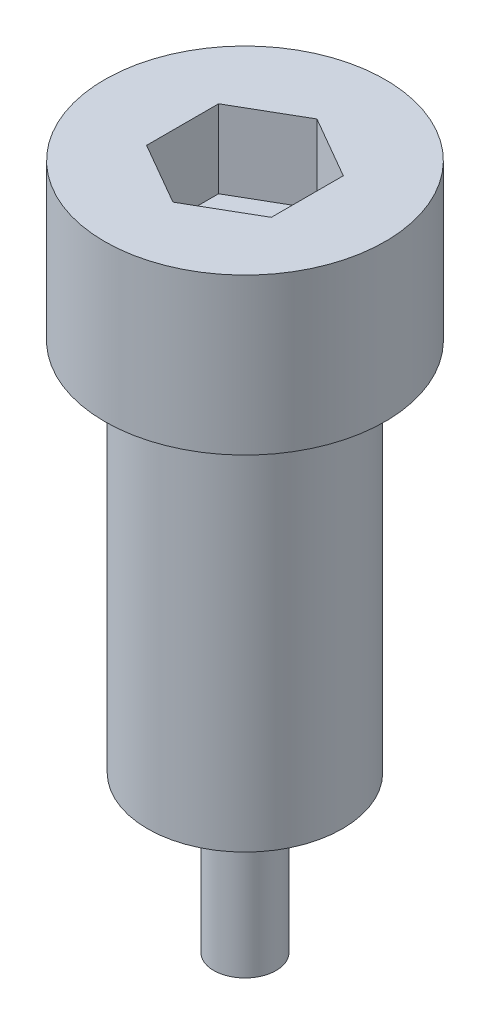
from build123d import *

# Parameters (mm, degrees)
SKETCH1_R           = 2
BOSS_EXTRUDE1_DEPTH = 10
SKETCH2_R           = 6.25
BOSS_EXTRUDE2_DEPTH = 24
SKETCH3_R           = 9
BOSS_EXTRUDE3_DEPTH = 10
CUT_EXTRUDE1_DEPTH  = 5


with BuildPart() as part:
    # Sketch1 → Boss-Extrude1 (new body)
    with BuildSketch(Plane(origin=(0, 0, 0), x_dir=(1, 0, 0), z_dir=(0, 1, 0))):
        with Locations(Location((0, 0, 0), (0, 0, 270))):
            Circle(SKETCH1_R)
    extrude(amount=BOSS_EXTRUDE1_DEPTH)

    # Sketch2 → Boss-Extrude2 (add)
    with BuildSketch(Plane(origin=(0, 10, 0), x_dir=(1, 0, 0), z_dir=(0, 1, 0))):
        with Locations(Location((0, 0, 0), (0, 0, 270))):
            Circle(SKETCH2_R)
    extrude(amount=BOSS_EXTRUDE2_DEPTH)

    # Sketch3 → Boss-Extrude3 (add)
    with BuildSketch(Plane(origin=(0, 34, 0), x_dir=(1, 0, 0), z_dir=(0, 1, 0))):
        with Locations(Location((0, 0, 0), (0, 0, 270))):
            Circle(SKETCH3_R)
    extrude(amount=BOSS_EXTRUDE3_DEPTH)

    # Sketch4 → Cut-Extrude1 (cut)
    with BuildSketch(Plane(origin=(0, 44, 0), x_dir=(1, 0, 0), z_dir=(0, 1, 0))):
        Polygon((0, 4.618802154), (-4, 2.309401077), (-4, -2.309401077), (0, -4.618802154), (4, -2.309401077), (4, 2.309401077), align=None)
    extrude(amount=-CUT_EXTRUDE1_DEPTH, mode=Mode.SUBTRACT)


solid = part.part
